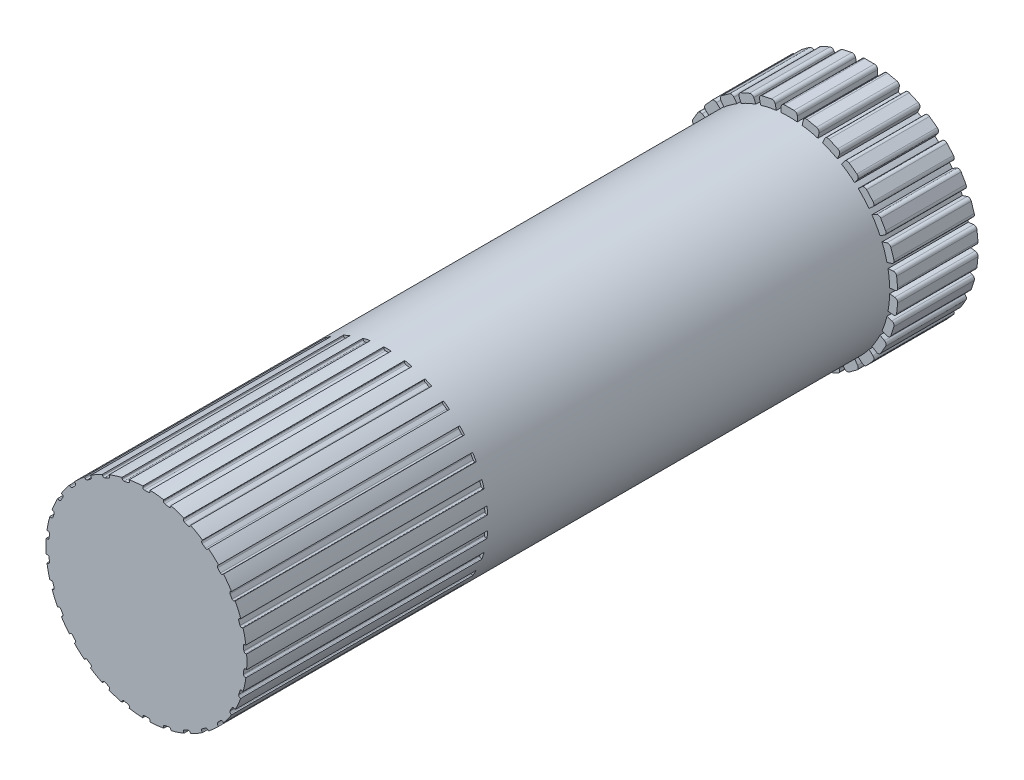
from build123d import *

# Parameters (mm, degrees)
SKETCH1_R           = 12.5
BOSS_EXTRUDE1_DEPTH = 90
CUT_EXTRUDE1_DEPTH  = 30
CIRPATTERN1_COUNT   = 30
BOSS_EXTRUDE2_DEPTH = 10
CIRPATTERN4_COUNT   = 30


with BuildPart() as part:
    # Sketch1 → Boss-Extrude1 (new body)
    with BuildSketch(Plane.XY):
        with Locations(Location((0, 0, 0), (0, 0, 180))):
            Circle(SKETCH1_R)
    extrude(amount=BOSS_EXTRUDE1_DEPTH)

    # Sketch3 → Cut-Extrude1 (cut)
    with BuildSketch(Plane.XY.offset(90)):
        with BuildLine():
            Line((-0.457592357, 12.840207999), (0.457592357, 12.840207999))
            Line((0.457592357, 12.840207999), (0.457592357, 12.359792001))
            ThreePointArc((0.457592357, 12.359792001), (0.399013713, 12.218370645), (0.257592357, 12.159792001))
            Line((0.257592357, 12.159792001), (-0.257592357, 12.159792001))
            ThreePointArc((-0.257592357, 12.159792001), (-0.399013713, 12.218370645), (-0.457592357, 12.359792001))
            Line((-0.457592357, 12.359792001), (-0.457592357, 12.840207999))
        make_face()
    cut_extrude1 = extrude(amount=-CUT_EXTRUDE1_DEPTH, mode=Mode.SUBTRACT)

    # CirPattern1: Cut-Extrude1 ×30 about axis
    cirpattern1_axis = Axis((0, 0, 0), (0, 0, 1))
    for i in range(1, CIRPATTERN1_COUNT):
        add(cut_extrude1.rotate(cirpattern1_axis, i * 360 / CIRPATTERN1_COUNT), mode=Mode.SUBTRACT)

    # Sketch6 → Boss-Extrude2 (add)
    with BuildSketch(Plane(origin=(0, 0, 0), x_dir=(-1, 0, 0), z_dir=(0, 0, -1))):
        with BuildLine():
            Line((-0.6, 13.5), (0.6, 13.5))
            ThreePointArc((0.6, 13.5), (0.882842712, 13.382842712), (1, 13.1))
            Line((1, 13.1), (1, 11.9))
            ThreePointArc((1, 11.9), (0.882842712, 11.617157288), (0.6, 11.5))
            Line((0.6, 11.5), (-0.6, 11.5))
            ThreePointArc((-0.6, 11.5), (-0.882842712, 11.617157288), (-1, 11.9))
            Line((-1, 11.9), (-1, 13.1))
            ThreePointArc((-1, 13.1), (-0.882842712, 13.382842712), (-0.6, 13.5))
        make_face()
    boss_extrude2 = extrude(amount=-BOSS_EXTRUDE2_DEPTH)

    # CirPattern4: Boss-Extrude2 ×30 about axis
    cirpattern4_axis = Axis((0, 0, 0), (0, 0, 1))
    for i in range(1, CIRPATTERN4_COUNT):
        add(boss_extrude2.rotate(cirpattern4_axis, i * 360 / CIRPATTERN4_COUNT))


solid = part.part
